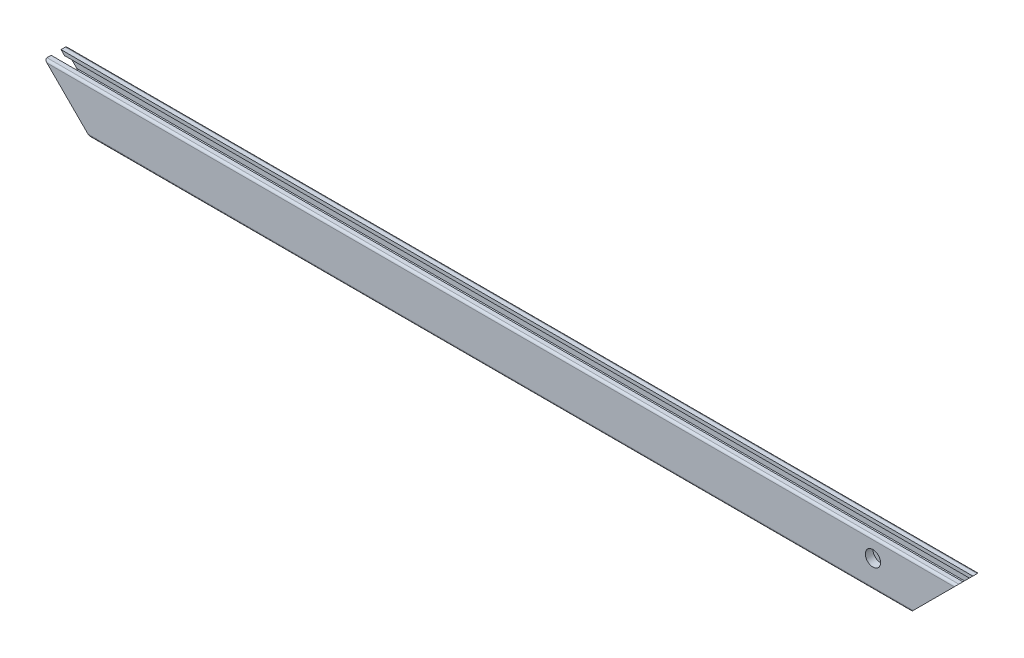
from build123d import *

# Parameters (mm, degrees)
SKETCH12_R          = 2.5
MEMBER_1_DEPTH      = 600
CUT_EXTRUDE_1_DEPTH = 301.749064836
SKETCH_7_R          = 5
CUT_EXTRUDE_2_DEPTH = 4.999


with BuildPart() as part:
    # Sketch12 → Member 1 (new body)
    with BuildSketch(Plane(origin=(-300, 0, 0), x_dir=(0, 0, -1), z_dir=(1, 0, 0))):
        with BuildLine():
            Line((-6, -15), (-3.25, -15))
            Line((-3.25, -15), (-3.25, -12.7))
            Line((-3.25, -12.7), (-5.7, -12.7))
            Line((-5.7, -12.7), (-5.7, -7))
            ThreePointArc((-5.7, -7), (0, -4.5), (5.7, -7))
            Line((5.7, -7), (5.7, -12.7))
            Line((5.7, -12.7), (3.25, -12.7))
            Line((3.25, -12.7), (3.25, -15))
            Line((3.25, -15), (6, -15))
            ThreePointArc((6, -15), (7.060660172, -14.560660172), (7.5, -13.5))
            Line((7.5, -13.5), (7.5, 13.5))
            ThreePointArc((7.5, 13.5), (7.060660172, 14.560660172), (6, 15))
            Line((6, 15), (3.25, 15))
            Line((3.25, 15), (3.25, 12.7))
            Line((3.25, 12.7), (5.7, 12.7))
            Line((5.7, 12.7), (5.7, 7))
            ThreePointArc((5.7, 7), (0, 4.5), (-5.7, 7))
            Line((-5.7, 7), (-5.7, 12.7))
            Line((-5.7, 12.7), (-3.25, 12.7))
            Line((-3.25, 12.7), (-3.25, 15))
            Line((-3.25, 15), (-6, 15))
            ThreePointArc((-6, 15), (-7.060660172, 14.560660172), (-7.5, 13.5))
            Line((-7.5, 13.5), (-7.5, -13.5))
            ThreePointArc((-7.5, -13.5), (-7.060660172, -14.560660172), (-6, -15))
        make_face()
        Circle(SKETCH12_R, mode=Mode.SUBTRACT)
    extrude(amount=MEMBER_1_DEPTH)

    # 草图4 → 切除-拉伸1 (cut, through all)
    with BuildSketch(Plane.XY.offset(7.5)):
        Polygon((-300, 15), (-270, -15), (-300, -15), align=None)
        Polygon((300, -15), (300, 15), (270, -15), align=None)
    extrude(amount=-CUT_EXTRUDE_1_DEPTH, mode=Mode.SUBTRACT)

    # 草图7 → 切除-拉伸2 (cut)
    with BuildSketch(Plane.XY.offset(7.5)):
        with Locations((245, 3)):
            Circle(SKETCH_7_R)
    extrude(amount=-CUT_EXTRUDE_2_DEPTH, mode=Mode.SUBTRACT)


solid = part.part
